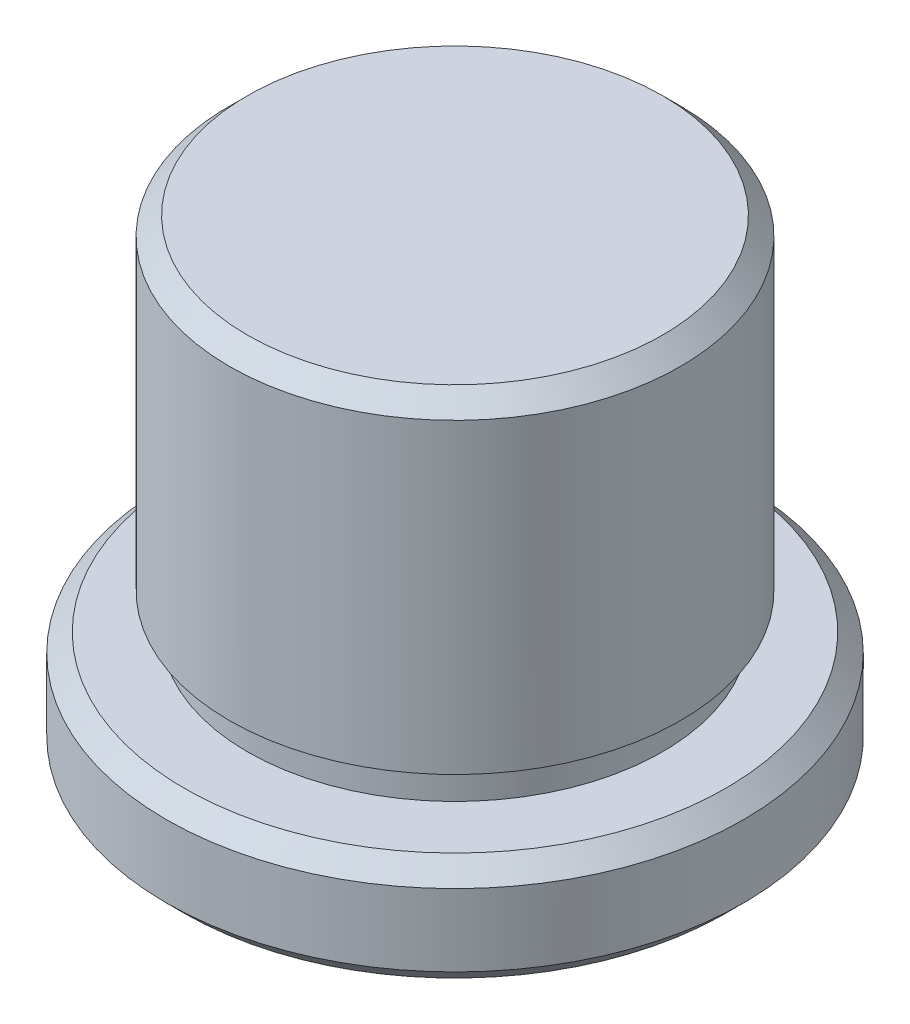
SolidWorks part; units mm, degrees
material "20"
ref_plane "Front Plane" through (0, 0, 0) normal (0, 0, 1) x (1, 0, 0)
ref_plane "Top Plane" through (0, 0, 0) normal (0, 1, 0) x (1, 0, 0)
ref_plane "Right Plane" through (0, 0, 0) normal (1, 0, 0) x (0, 0, -1)
sketch "Sketch1" plane through (0, 0, 0) normal (0, 0, 1) x (1, 0, 0)
  line L0 (67.7737, -120.8) -> (67.7737, -125.3) construction
  line L1 (80.2737, -128.5) -> (80.2737, -125.3) construction
  line L2 (74.0237, -131.5) -> (74.0237, -118.5)
  line L4 (82.0237, -128.5) -> (79.7737, -128.5)
  line L5 (83.1526, -128.5) -> (86.6881, -128.5) construction
  line L6 (82.0237, -128.5) -> (82.0237, -131.5)
  line L7 (74.0237, -118.5) -> (74.0237, -131.5) construction
  line L8 (80.2737, -127.5) -> (80.2737, -118.5)
  line L10 (82.0237, -131.5) -> (74.0237, -131.5)
  line L11 (80.2737, -118.5) -> (74.0237, -118.5)
  line L13 (80.2737, -127.5) -> (79.7737, -127.5)
  line L14 (79.7737, -127.5) -> (79.7737, -128.5)
  line L15 (83.1526, -128.5) -> (61.0237, -128.5) construction
  dimension "D1" = 6.25
  dimension "D2" = 3
  dimension "D3" = 16
  dimension "D4" = 0.5
  dimension "D5" = 1
  dimension "D6" = 9
revolve "Revolve1" add sketch "Sketch1" angle 360 about L7
chamfer "Chamfer1" distance 0.5 angle 45 3 edges at (74.0237, -128.5, 8) (74.0237, -131.5, 8) (74.0237, -118.5, 6.25)
